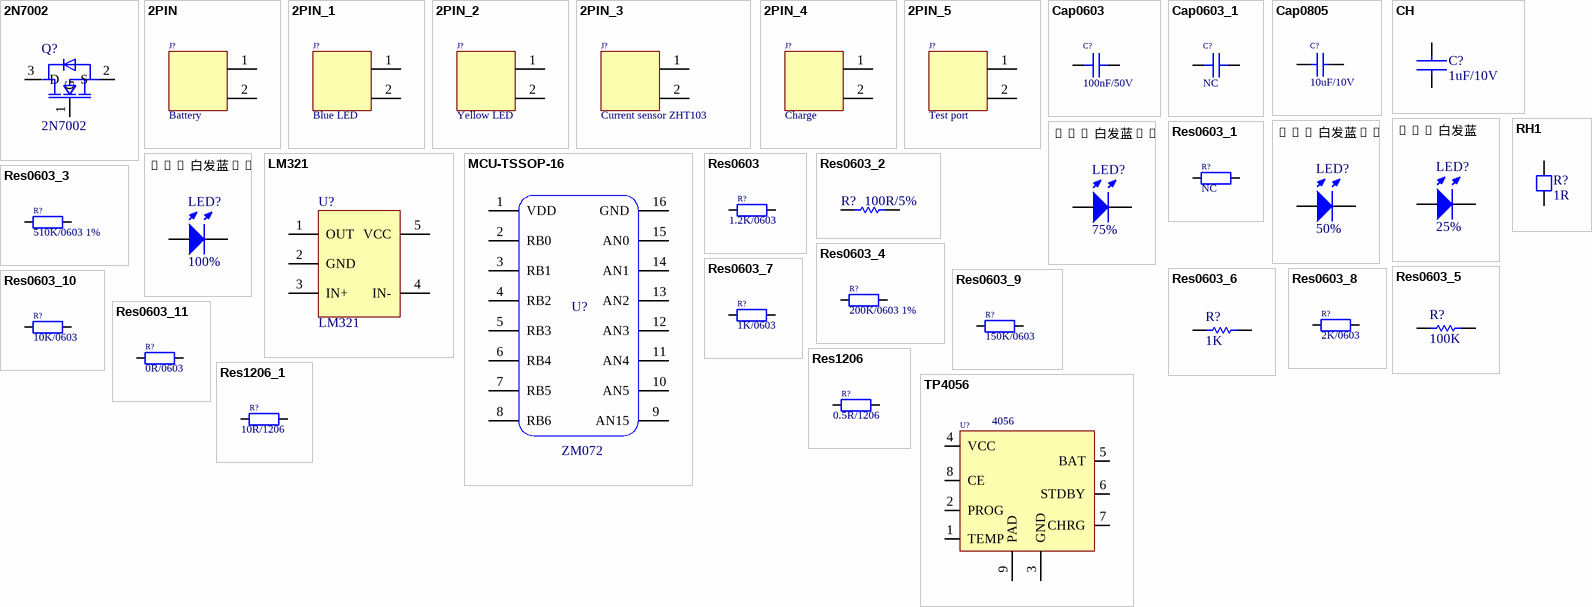
[diagram p0: symbols 2N7002 to TP4056]
# Altium schematic symbol library MISC75737-4.SchLib: 33 symbols
Pins are listed as number, name and electrical type; pins without a type are passive.


## 2N7002
designator Q?
SMD MOS
footprint SOT23-3L (SMD MOS)
footprint SOT23-3 (SMD IC/MOS*)
pins: 1 G, 2 S, 3 D

## 2PIN
designator J?, comment Battery
DC socket right-angle 90° pitch 2.0; 物料名称: DC socket 2PIN; 封装: Pitch 2.0 90° right-angle THT
footprint GH1.25-2PIN立贴带扣耐温260℃ (Vertical SMD with latch, rated 260℃)
pins: 1, 2

## 2PIN_1
designator J?, comment Blue LED
DC socket right-angle 90° pitch 2.0; 物料名称: DC socket 2PIN; 封装: Pitch 2.0 90° right-angle THT
footprint GH1.25-2PIN立贴带扣耐温260℃ (Vertical SMD with latch, rated 260℃)
pins: 1, 2

## 2PIN_2
designator J?, comment Yellow LED
DC socket right-angle 90° pitch 2.0; 物料名称: DC socket 2PIN; 封装: Pitch 2.0 90° right-angle THT
footprint GH1.25-2PIN立贴带扣耐温260℃ (Vertical SMD with latch, rated 260℃)
pins: 1, 2

## 2PIN_3
designator J?, comment Current sensor ZHT103
DC socket right-angle 90° pitch 2.0; 物料名称: DC socket 2PIN; 封装: Pitch 2.0 90° right-angle THT
footprint IND-TH_L18.2-W10.2-P12.00-D0.9_ZHT103
pins: 1, 2

## 2PIN_4
designator J?, comment Charge
DC socket right-angle 90° pitch 2.0; 物料名称: DC socket 2PIN; 封装: Pitch 2.0 90° right-angle THT
footprint HY2.0WT-2A/P 立贴带扣耐温260℃ (Horizontal SMD connector)
pins: 1, 2

## 2PIN_5
designator J?, comment Test port
DC socket right-angle 90° pitch 2.0; 物料名称: DC socket 2PIN; 封装: Pitch 2.0 90° right-angle THT
footprint HY2.0WT-2A/P 立贴带扣耐温260℃ (Horizontal SMD connector)
pins: 1, 2

## Cap0603
designator C?, comment 100nF/50V
footprint C0603A (SMD capacitor)
pins: 1, 2

## Cap0603_1
designator C?, comment NC
footprint C0603A (SMD capacitor)
pins: 1, 2

## Cap0805
designator C?, comment 10uF/10V
SMD capacitor; 规格: 0805-16V-106-X7R
footprint C0805 (SMD capacitor C0805)
footprint C0805A (SMD capacitor)
pins: 1, 2

## CH
designator C?, comment 1uF/10V
footprint 0603HD
footprint 0805B
footprint 1206H
footprint 0603C
footprint 0603DC
footprint C0603A (SMD capacitor)
pins: 1, 2
2 alternate drawings of the same symbol

## LED 白发蓝
designator LED?, comment 25%
SMD LED; 规格: 0603-diffused-ice blue
footprint 0603-LED-CB
footprint LED-DIP-2
footprint LED0603A
footprint LED-0603
footprint 0603-LED
footprint LED0603A (SMD LED)
pins: 1, 2

## LED 白发蓝_1
designator LED?, comment 50%
SMD LED; 规格: 0603-diffused-ice blue
footprint 0603-LED-CB
footprint LED-DIP-2
footprint LED0603A
footprint LED-0603
footprint 0603-LED
footprint LED0603A (SMD LED)
pins: 1, 2

## LED 白发蓝_2
designator LED?, comment 75%
SMD LED; 规格: 0603-diffused-ice blue
footprint 0603-LED-CB
footprint LED-DIP-2
footprint LED0603A
footprint LED-0603
footprint 0603-LED
footprint LED0603A (SMD LED)
pins: 1, 2

## LED 白发蓝_3
designator LED?, comment 100%
SMD LED; 规格: 0603-diffused-ice blue
footprint 0603-LED-CB
footprint LED-DIP-2
footprint LED0603A
footprint LED-0603
footprint 0603-LED
footprint LED0603A (SMD LED)
pins: 1, 2

## LM321
designator U?
footprint SOT-23-5
footprint SOT23-5A (SMD IC)
pins: 1 OUT, 2 GND, 3 IN+, 4 IN-, 5 VCC

## MCU-TSSOP-16
designator U?, comment ZM072
footprint TSSOP-20
footprint TSSOP-16A
footprint TSSOP-16(间距0.65mm) (SMD IC)
footprint SOP16L
pins: 1 VDD, 2 RB0, 3 RB1, 4 RB2, 5 RB3, 6 RB4, 7 RB5, 8 RB6, 9 AN15, 10 AN5, 11 AN4, 12 AN3, 13 AN2, 14 AN1, 15 AN0, 16 GND

## Res0603
designator R?, comment 1.2K/0603
SMD resistor; 规格: 0603
footprint R0603
footprint R0603A (SMD resistor)
pins: 1, 2

## Res0603_1
designator R?, comment NC
SMD resistor; 规格: 0603
footprint R0603
footprint R0603A (SMD resistor)
pins: 1, 2

## Res0603_2
designator R?, comment 100R/5%
SMD resistor; 规格: 0603
footprint 0603 (1608)
footprint 0402 (1005)
footprint 1206 (3216)
footprint 2512 (6432)
footprint 0201 (0603)
footprint 0805 (2012)
footprint 1210 (3528  3225)
footprint R0603
footprint R0603
footprint 0603D
footprint R0603A (SMD resistor)
pins: 1, 2

## Res0603_3
designator R?, comment 510K/0603 1%
SMD resistor; 规格: 0603
footprint R0603
footprint R0603A (SMD resistor)
pins: 1, 2

## Res0603_4
designator R?, comment 200K/0603 1%
SMD resistor; 规格: 0603
footprint R0603
footprint R0603A (SMD resistor)
pins: 1, 2

## Res0603_5
designator R?, comment 100K
SMD resistor; 规格: 0603
footprint 0603 (1608)
footprint 0402 (1005)
footprint 1206 (3216)
footprint 2512 (6432)
footprint 0201 (0603)
footprint 0805 (2012)
footprint 1210 (3528  3225)
footprint R0603
footprint R0603
footprint 0603D
footprint R0603A (SMD resistor)
pins: 1, 2

## Res0603_6
designator R?, comment 1K
SMD resistor; 规格: 0603
footprint 0603 (1608)
footprint 0402 (1005)
footprint 1206 (3216)
footprint 2512 (6432)
footprint 0201 (0603)
footprint 0805 (2012)
footprint 1210 (3528  3225)
footprint R0603
footprint R0603
footprint 0603D
footprint R0603A (SMD resistor)
pins: 1, 2

## Res0603_7
designator R?, comment 1K/0603
SMD resistor; 规格: 0603
footprint R0603
footprint R0603A (SMD resistor)
pins: 1, 2

## Res0603_8
designator R?, comment 2K/0603
SMD resistor; 规格: 0603
footprint R0603
footprint R0603A (SMD resistor)
pins: 1, 2

## Res0603_9
designator R?, comment 150K/0603
SMD resistor; 规格: 0603
footprint R0603
footprint R0603A (SMD resistor)
pins: 1, 2

## Res0603_10
designator R?, comment 10K/0603
SMD resistor; 规格: 0603
footprint R0603
footprint R0603A (SMD resistor)
pins: 1, 2

## Res0603_11
designator R?, comment 0R/0603
SMD resistor; 规格: 0603
footprint R0603
footprint R0603A (SMD resistor)
pins: 1, 2

## Res1206
designator R?, comment 0.5R/1206
SMD resistor; 规格: 0603-43.2K-1%
footprint R1206
footprint R1206A (SMD resistor)
pins: 1, 2

## Res1206_1
designator R?, comment 10R/1206
SMD resistor; 规格: 0603-43.2K-1%
footprint R1206
footprint R1206A (SMD resistor)
pins: 1, 2

## RH1
designator R?, comment 1R
footprint 0603D
footprint 0805H
footprint 1206H
footprint 0603C
footprint R0603A (SMD resistor)
pins: 1, 2
2 alternate drawings of the same symbol

## TP4056
designator U?, comment 4056
Charger IC; 规格: ESOP-8; 物料名称: Charger IC 4056
footprint ESOP-8
footprint ESOP-8L (SMD MOS/IC)
pins: 1 TEMP, 2 PROG, 3 GND, 4 VCC, 5 BAT, 6 STDBY, 7 CHRG, 8 CE, 9 PAD